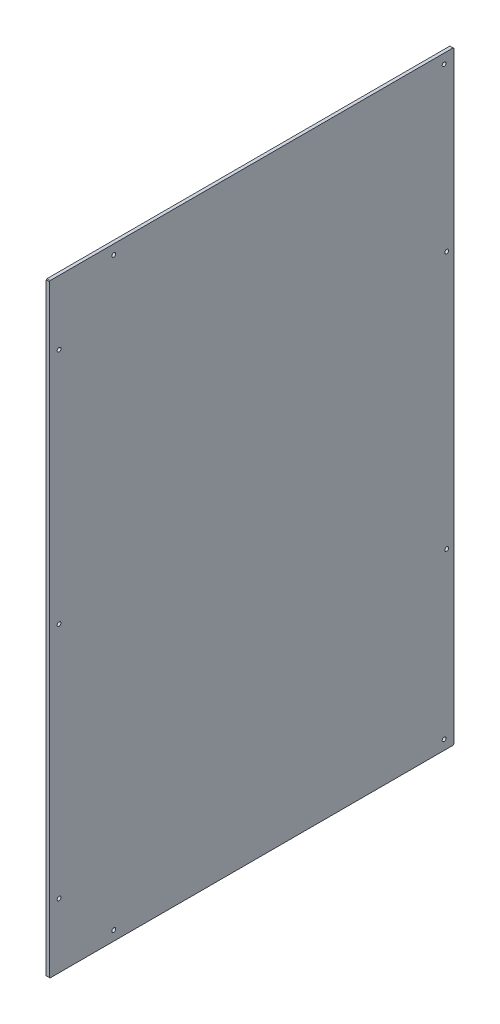
SolidWorks part; units mm, degrees
material "PC(透明)"
ref_plane "前基準面" through (0, 0, 0) normal (0, 0, 1) x (1, 0, 0)
ref_plane "上基準面" through (0, 0, 0) normal (0, 1, 0) x (1, 0, 0)
ref_plane "右基準面" through (0, 0, 0) normal (1, 0, 0) x (0, 0, -1)
sketch "草图1" plane through (0, 0, 0) normal (1, 0, 0) x (0, 0, -1)
  line L1 (314, 469) -> (-314, 469)
  line L2 (314, 469) -> (314, -469)
  line L3 (314, -469) -> (-314, -469)
  line L4 (-314, 469) -> (-314, -469)
  line L5 (314, 469) -> (-314, -469) construction
  line L6 (314, -469) -> (-314, 469) construction
  point P0 (0, 0)
  dimension "D1" = 628
  dimension "D2" = 938
extrude "凸台-拉伸1" add sketch "草图1" along normal blind 5
chamfer "倒角1" distance 1 angle 45 4 edges at (2.5, -469, -314) (2.5, -469, 314) (2.5, 469, -314) (2.5, 469, 314)
sketch "草图2" plane through (0, 0, 0) normal (-1, 0, 0) x (0, 0, 1)
  line L0 (-303, 200) -> (-303, -200) construction
  line L1 (-313, 469) -> (313, 469) construction
  line L2 (58.8862, 0) -> (0, 0) construction
  line L3 (0, 0) -> (0, 69.8386) construction
  line L4 (314, 468) -> (314, -468) construction
  line L5 (299, -454) -> (-299, -454) construction
  line L6 (299, -454) -> (299, 454) construction
  line L7 (299, 454) -> (-299, 454) construction
  line L8 (-299, -454) -> (-299, 454) construction
  line L9 (299, -454) -> (-299, 454) construction
  line L10 (299, 454) -> (-299, -454) construction
  line L11 (-313, 469) -> (313, 469) construction
  line L12 (313, -469) -> (-313, -469) construction
  line L13 (-314, -468) -> (-314, 468) construction
  line L14 (-303, 0) -> (-314, 0) construction
  circle A0 centre (-299, 454) radius 3
  circle A1 centre (-299, -454) radius 3
  circle A2 centre (299, -454) radius 3 construction
  circle A3 centre (299, 454) radius 3 construction
  circle A4 centre (214, 454) radius 3
  circle A5 centre (299, 369) radius 3
  circle A6 centre (299, -369) radius 3
  circle A7 centre (214, -454) radius 3
  circle A8 centre (299, 0) radius 3
  circle A9 centre (-299, 0) radius 3 construction
  circle A10 centre (-303, 200) radius 3
  circle A11 centre (-303, -200) radius 3
  dimension "D1" = 6
  dimension "D4" = 100
  dimension "D5" = 100
  dimension "D2" = 15
  dimension "D3" = 15
  dimension "D6" = 100
  dimension "D7" = 15
  dimension "D8" = 11
  dimension "D9" = 400
extrude "切除-拉伸1" cut sketch "草图2" against normal through all
